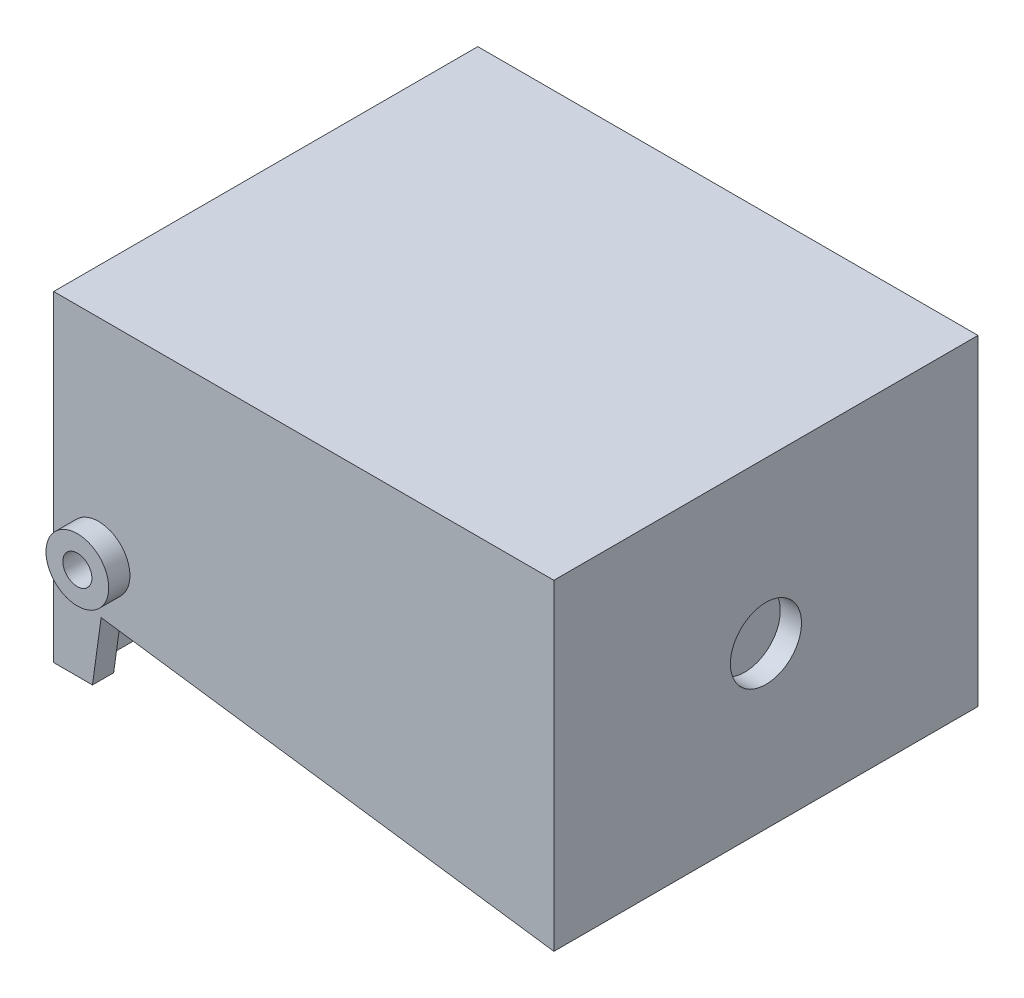
from build123d import *

# Parameters (mm, degrees)
SKETCH1_W               = 11.793584223
SKETCH1_H               = 7.577709462
BOSS_EXTRUDE1_DEPTH     = 10
SHELL1_T                = -0.5
CUT_EXTRUDE1_DEPTH      = 47.145900644
CUT_EXTRUDE1_DEPTH_BACK = 47.145900644
SKETCH3_R               = 0.739402186
BOSS_EXTRUDE2_DEPTH     = 0.5
CUT_EXTRUDE2_DEPTH      = 47.256828104
CUT_EXTRUDE2_DEPTH_BACK = 47.256828104
SKETCH4_R               = 0.342163572
CUT_EXTRUDE3_DEPTH      = 18.219474717
CUT_EXTRUDE3_DEPTH_BACK = 0.5
SKETCH5_R               = 0.838133872
SKETCH6_R               = 1.176594154
BOSS_EXTRUDE3_DEPTH     = 1.5
SKETCH7_R               = 2
BOSS_EXTRUDE4_DEPTH     = 3
SKETCH8_R               = 2.5
BOSS_EXTRUDE5_DEPTH     = 3
SKETCH9_R               = 2.944420976
BOSS_EXTRUDE6_DEPTH     = 3.293584224


with BuildPart() as part:
    # Sketch1 → Boss-Extrude1 (new body)
    with BuildSketch(Plane.XY):
        with Locations((-38.510667459, -3.788854731)):
            Rectangle(SKETCH1_W, SKETCH1_H)
    extrude(amount=-BOSS_EXTRUDE1_DEPTH)

    # Shell1
    shell1_openings = [part.faces().sort_by_distance(p)[0] for p in [
        (-38.510667459, -7.577709462, -5),
    ]]
    offset(amount=SHELL1_T, openings=shell1_openings, kind=Kind.INTERSECTION)

    # Sketch2 → Cut-Extrude1 (cut, two sides: drawn at the far end of the back side and taken through both)
    with BuildSketch(Plane.XY.offset(-CUT_EXTRUDE1_DEPTH_BACK)):
        Polygon((-32.613875348, -7.577709462), (-43.28798944, -6.09867093), (-43.492929631, -7.577709462), (-42.32222074, -12.914238607), (-34.209763667, -9.465064681), align=None)
    extrude(amount=CUT_EXTRUDE1_DEPTH + CUT_EXTRUDE1_DEPTH_BACK, mode=Mode.SUBTRACT)

    # Sketch3 → Boss-Extrude2 (add)
    with BuildSketch(Plane.XY):
        with Locations(Location((-43.348851562, -4.90387791, 0), (0, 0, 180))):
            Circle(SKETCH3_R)
    extrude(amount=BOSS_EXTRUDE2_DEPTH)

    # Sketch4 → Cut-Extrude2 (cut, two sides: drawn at the far end of the back side and taken through both)
    with BuildSketch(Plane.XY.offset(0.5).offset(-CUT_EXTRUDE2_DEPTH_BACK)):
        with Locations((-43.348851562, -4.90387791)):
            Circle(SKETCH4_R)
    extrude(amount=CUT_EXTRUDE2_DEPTH + CUT_EXTRUDE2_DEPTH_BACK, mode=Mode.SUBTRACT)

    # Sketch5 → Cut-Extrude3 (cut, two sides: drawn at the far end of the back side and taken through both)
    with BuildSketch(Plane(origin=(-32.613875348, 0, 0), x_dir=(0, 0, -1), z_dir=(1, 0, 0)).offset(-CUT_EXTRUDE3_DEPTH_BACK)):
        with Locations(Location((5, -3.788854731, 0), (0, 0, 180))):
            Circle(SKETCH5_R)
    extrude(amount=CUT_EXTRUDE3_DEPTH + CUT_EXTRUDE3_DEPTH_BACK, mode=Mode.SUBTRACT)

    # Sketch6 → Boss-Extrude3 (add)
    with BuildSketch(Plane(origin=(-43.907459571, 0, 0), x_dir=(0, 0, -1), z_dir=(1, 0, 0))):
        with Locations(Location((5, -4.038854731, 0), (0, 0, 180))):
            Circle(SKETCH6_R)
    extrude(amount=BOSS_EXTRUDE3_DEPTH)

    # Sketch7 → Boss-Extrude4 (add)
    with BuildSketch(Plane(origin=(-42.407459571, 0, 0), x_dir=(0, 0, -1), z_dir=(1, 0, 0))):
        with Locations((5, -4.038854731)):
            Circle(SKETCH7_R)
    extrude(amount=BOSS_EXTRUDE4_DEPTH)

    # Sketch8 → Boss-Extrude5 (add)
    with BuildSketch(Plane(origin=(-39.407459571, 0, 0), x_dir=(0, 0, -1), z_dir=(1, 0, 0))):
        with Locations((5, -4.038854731)):
            Circle(SKETCH8_R)
    extrude(amount=BOSS_EXTRUDE5_DEPTH)

    # Sketch9 → Boss-Extrude6 (add)
    with BuildSketch(Plane(origin=(-36.407459571, 0, 0), x_dir=(0, 0, -1), z_dir=(1, 0, 0))):
        with Locations((5, -4.038854731)):
            Circle(SKETCH9_R)
    extrude(amount=BOSS_EXTRUDE6_DEPTH)


solid = part.part
